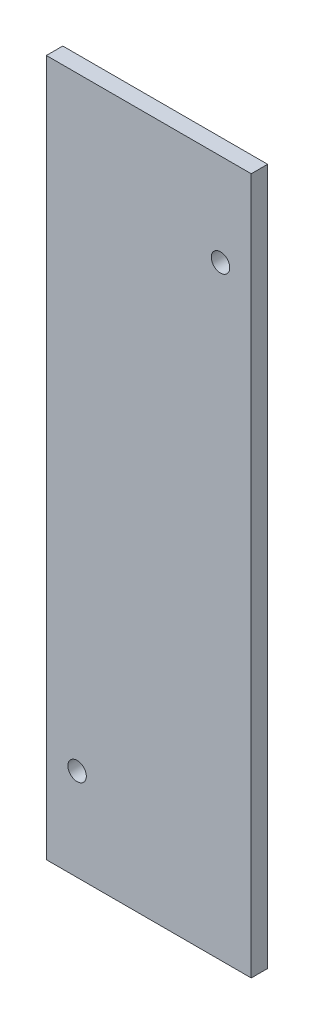
from build123d import *

# Parameters (mm, degrees)
SKETCH_1_W          = 100
SKETCH_1_H          = 340
EXTRUDE_1_DEPTH     = 4
SKETCH_2_R          = 4.5
CUT_EXTRUDE_1_DEPTH = 14


with BuildPart() as part:
    # 草图1 → 凸台-拉伸1 (new, symmetric)
    with BuildSketch(Plane.XY):
        Rectangle(SKETCH_1_W, SKETCH_1_H)
    extrude(amount=EXTRUDE_1_DEPTH, both=True)

    # 草图2 → 切除-拉伸1 (cut, symmetric)
    with BuildSketch(Plane.XY):
        with Locations((-35, -125)):
            Circle(SKETCH_2_R)
        with Locations((35, 125)):
            Circle(SKETCH_2_R)
    extrude(amount=CUT_EXTRUDE_1_DEPTH, both=True, mode=Mode.SUBTRACT)


solid = part.part
